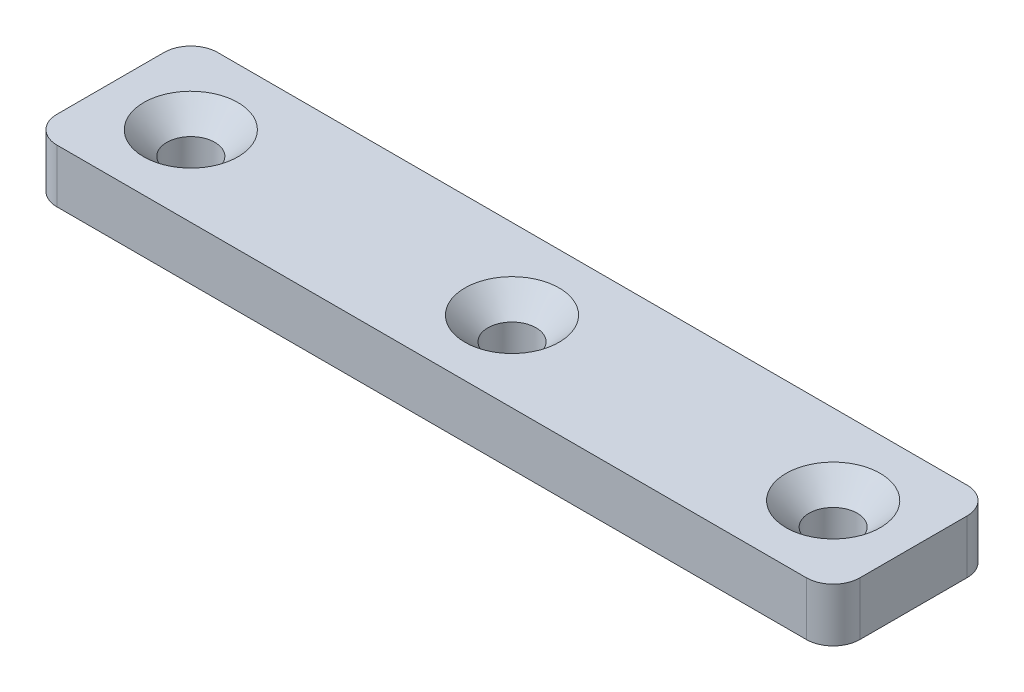
from build123d import *

# Parameters (mm, degrees)
SKETCH1_W                                  = 150
SKETCH1_H                                  = 30
BOSS_EXTRUDE1_DEPTH                        = 10
FILLET1_R                                  = 5
SOCKET_BUTTON_HEAD_SCREW_HOLE1_D           = 9
SOCKET_BUTTON_HEAD_SCREW_HOLE1_DEPTH       = 19.75
SOCKET_BUTTON_HEAD_SCREW_HOLE1_CSINK_D     = 17.6
SOCKET_BUTTON_HEAD_SCREW_HOLE1_CSINK_ANGLE = 90
SOCKET_BUTTON_HEAD_SCREW_HOLE1_TIP         = 2.703872786


with BuildPart() as part:
    # Sketch1 → Boss-Extrude1 (new body)
    with BuildSketch(Plane(origin=(0, 0, 0), x_dir=(1, 0, 0), z_dir=(0, 1, 0))):
        with Locations((75, 15)):
            Rectangle(SKETCH1_W, SKETCH1_H)
    extrude(amount=BOSS_EXTRUDE1_DEPTH)

    # Fillet1
    fillet1_edges = [part.edges().sort_by_distance(p)[0] for p in [
        (0, 5, -30),
        (150, 5, -30),
        (150, 5, 0),
        (0, 5, 0),
    ]]
    fillet(fillet1_edges, radius=FILLET1_R)

    # Socket Button Head Screw Hole1
    with Locations(Plane(origin=(0, 10, 0), x_dir=(1, 0, 0), z_dir=(0, 1, 0))):
        with Locations((75, 15), (15, 15), (135, 15)):
            CounterSinkHole(SOCKET_BUTTON_HEAD_SCREW_HOLE1_D / 2, SOCKET_BUTTON_HEAD_SCREW_HOLE1_CSINK_D / 2, depth=SOCKET_BUTTON_HEAD_SCREW_HOLE1_DEPTH, counter_sink_angle=SOCKET_BUTTON_HEAD_SCREW_HOLE1_CSINK_ANGLE)
            with Locations((0, 0, -(SOCKET_BUTTON_HEAD_SCREW_HOLE1_DEPTH + SOCKET_BUTTON_HEAD_SCREW_HOLE1_TIP / 2))):  # 118° drill point
                Cone(0, SOCKET_BUTTON_HEAD_SCREW_HOLE1_D / 2, SOCKET_BUTTON_HEAD_SCREW_HOLE1_TIP, mode=Mode.SUBTRACT)


solid = part.part
